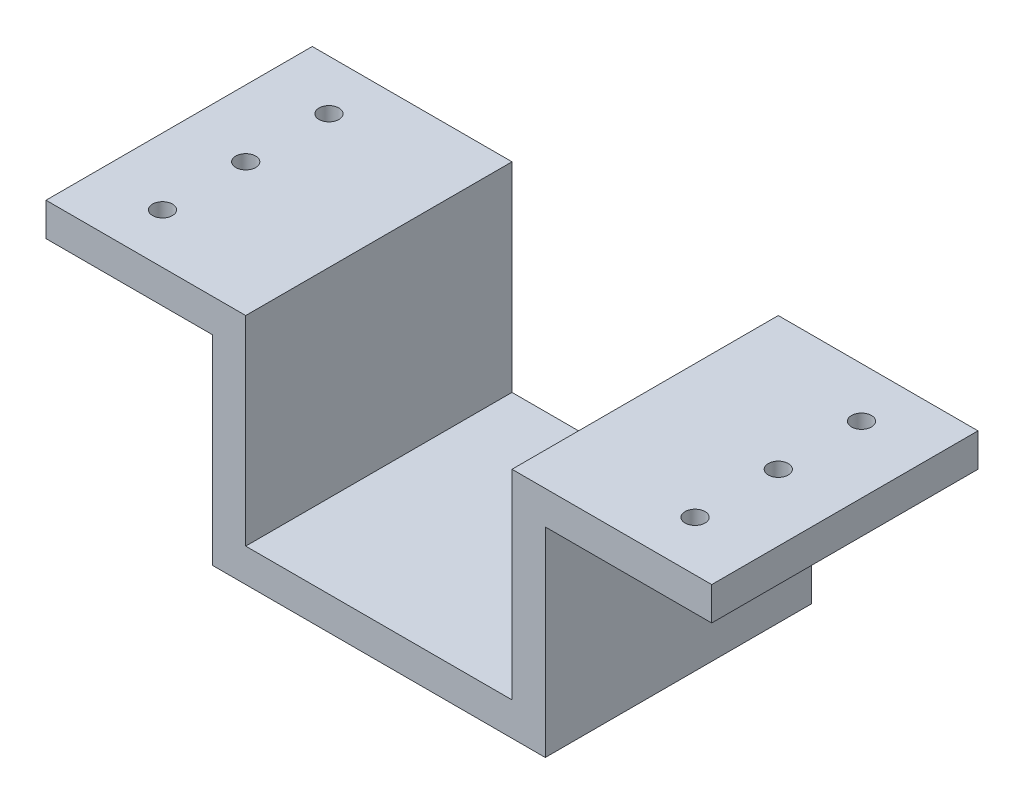
SolidWorks part; units mm, degrees
ref_plane "Front Plane" through (0, 0, 0) normal (0, 0, 1) x (1, 0, 0)
ref_plane "Top Plane" through (0, 0, 0) normal (0, 1, 0) x (1, 0, 0)
ref_plane "Right Plane" through (0, 0, 0) normal (1, 0, 0) x (0, 0, -1)
other "Configuration Table"
sketch "Sketch1" plane through (0, 0, 0) normal (0, 0, 1) x (1, 0, 0)
  line L0 (0, 0) -> (0, 55.2027) construction
  line L1 (0, 0) -> (-25, 0)
  line L2 (-25, 0) -> (-25, 30)
  line L3 (-25, 30) -> (-50, 30)
  line L4 (0, 5) -> (-20, 5)
  line L5 (-20, 5) -> (-20, 35)
  line L6 (-20, 35) -> (-50, 35)
  line L7 (-50, 35) -> (-50, 30)
  line L8 (50, 35) -> (50, 30)
  line L9 (20, 35) -> (50, 35)
  line L10 (20, 5) -> (20, 35)
  line L11 (0, 5) -> (20, 5)
  line L12 (25, 30) -> (50, 30)
  line L13 (25, 0) -> (25, 30)
  line L14 (0, 0) -> (25, 0)
  dimension "D2" = 40
  dimension "D3" = 25
  dimension "D4" = 30
  dimension "D1" = 5
extrude "Boss-Extrude1" add sketch "Sketch1" along normal blind 40
sketch "Sketch2" plane through (0, 35, 0) normal (0, 1, 0) x (1, 0, 0)
  line L0 (-40, 0) -> (-40, -40) construction
  line L1 (-20, 0) -> (-50, 0) construction
  line L2 (-20, -40) -> (-50, -40) construction
  line L3 (40, 0) -> (40, -40) construction
  line L4 (50, 0) -> (20, 0) construction
  line L5 (50, -40) -> (20, -40) construction
  line L6 (40, -7.5) -> (-46.676, -7.5) construction
  line L7 (40, -20) -> (-50, -20) construction
  line L8 (40, -32.5) -> (-46.676, -32.5) construction
  line L9 (-50, -40) -> (-50, 0) construction
  line L10 (50, -40) -> (50, 0) construction
  circle A0 centre (-40, -7.5) radius 1.5
  circle A1 centre (-40, -20) radius 1.5
  circle A2 centre (-40, -32.5) radius 1.5
  circle A3 centre (40, -7.5) radius 1.5
  circle A4 centre (40, -20) radius 1.5
  circle A5 centre (40, -32.5) radius 1.5
  dimension "D5" = 3
  dimension "D1" = 25
  dimension "D2" = 12.5
  dimension "D3" = 10
  dimension "D4" = 10
extrude "Cut-Extrude1" cut sketch "Sketch2" against normal through all
